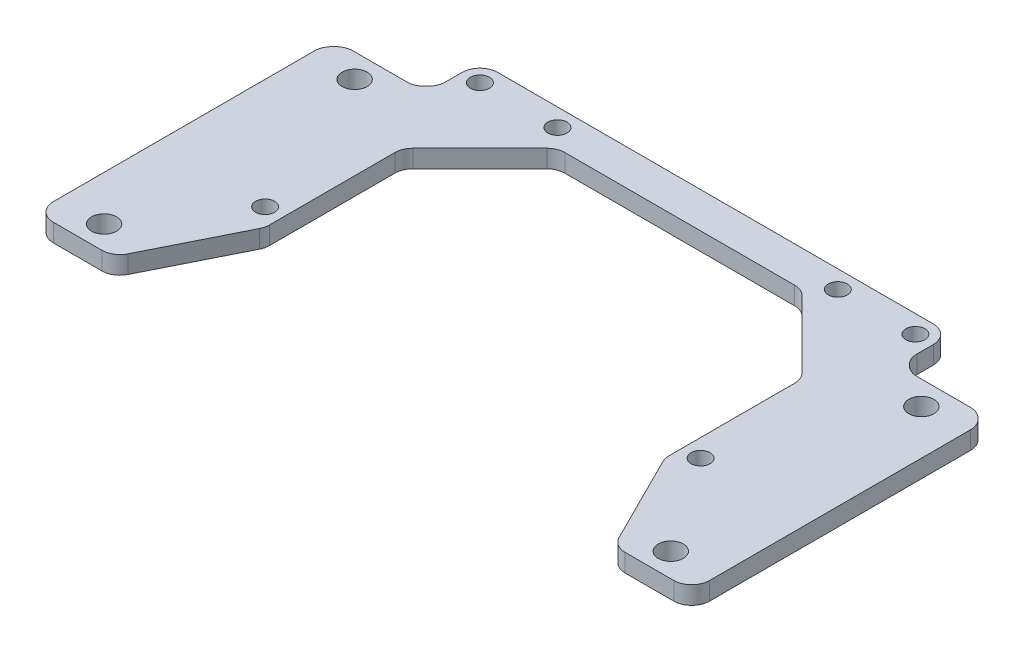
SolidWorks part; units mm, degrees
material "哈碳纤"
ref_plane "前视基准面" through (0, 0, 0) normal (0, 0, 1) x (1, 0, 0)
ref_plane "上视基准面" through (0, 0, 0) normal (0, 1, 0) x (1, 0, 0)
ref_plane "右视基准面" through (0, 0, 0) normal (1, 0, 0) x (0, 0, -1)
other "Configuration Table"
sketch "草图1" plane through (0, 0, 0) normal (0, 1, 0) x (1, 0, 0)
  line L0 (-23.5, 31) -> (23.5, 31) construction
  line L2 (-55, -25) -> (-55, 25)
  line L4 (55, -25) -> (55, 25)
  line L5 (-55, -25) -> (55, 25) construction
  line L6 (-55, 25) -> (55, -25) construction
  line L7 (-47.5, -21) -> (47.5, -21) construction
  line L8 (-47.5, -21) -> (-47.5, 21) construction
  line L9 (-47.5, 21) -> (47.5, 21) construction
  line L10 (47.5, -21) -> (47.5, 21) construction
  line L11 (-47.5, -21) -> (47.5, 21) construction
  line L12 (-47.5, 21) -> (47.5, -21) construction
  line L13 (-36.5, -5) -> (36.5, -5) construction
  line L14 (-36.5, -5) -> (-36.5, 31) construction
  line L15 (-36.5, 31) -> (36.5, 31) construction
  line L16 (36.5, -5) -> (36.5, 31) construction
  line L17 (-36.5, -5) -> (36.5, 31) construction
  line L18 (-36.5, 31) -> (36.5, -5) construction
  line L19 (0, -1000) -> (0, 49000) construction
  line L20 (-55, 25) -> (-39.5, 25)
  line L21 (55, 25) -> (39.5, 25)
  line L22 (-39.5, 25) -> (-39.5, 34)
  line L23 (39.5, 25) -> (39.5, 34)
  line L24 (-39.5, 34) -> (39.5, 34)
  line L25 (-55, -25) -> (-42, -25)
  line L26 (55, -25) -> (42, -25)
  line L27 (-42, -25) -> (-33.5, -8)
  line L28 (42, -25) -> (33.5, -8)
  line L29 (-33.5, -8) -> (-33.5, 28)
  line L30 (33.5, -8) -> (33.5, 28)
  line L31 (-33.5, 28) -> (0, 28)
  line L32 (33.5, 28) -> (0, 28)
  circle A0 centre (-47.5, 21) radius 2.1
  circle A1 centre (-47.5, -21) radius 2.1
  circle A2 centre (47.5, -21) radius 2.1
  circle A3 centre (47.5, 21) radius 2.1
  circle A4 centre (-36.5, 31) radius 1.6
  circle A5 centre (-36.5, -5) radius 1.6
  circle A6 centre (36.5, -5) radius 1.6
  circle A7 centre (36.5, 31) radius 1.6
  circle A8 centre (-23.5, 31) radius 1.6
  circle A9 centre (23.5, 31) radius 1.6
  point P0 (0, 0)
  point P5 (0, 0)
  point P15 (0, 13)
  point P28 (0, 31)
  point P36 (0, 34)
  dimension "D3" = 4.2
  dimension "D4" = 95
  dimension "D6" = 3.2
  dimension "D7" = 36
  dimension "D9" = 47
  dimension "D1" = 50
  dimension "D2" = 110
  dimension "D5" = 42
  dimension "D8" = 73
  dimension "D10" = 13
  dimension "D11" = 3
  dimension "D12" = 3
  dimension "D13" = 3
  dimension "D14" = 3
  dimension "D15" = 13
  dimension "D16" = 3
extrude "凸台-拉伸1" add sketch "草图1" along normal blind 3
chamfer "倒角1" distance 13 angle 45 2 edges at (33.5, 1.5, -28) (-33.5, 1.5, -28)
chamfer "倒角2" distance 2 angle 45 4 edges at (55, 1.5, -25) (39.5, 1.5, -25) (-55, 1.5, -25) (-39.5, 1.5, -25)
fillet "圆角1" radius 3 20 edges at (55, 1.5, 25) (42, 1.5, 25) (33.5, 1.5, 8) (33.5, 1.5, -15) (20.5, 1.5, -28) (-33.5, 1.5, -15) (-33.5, 1.5, 8) (-42, 1.5, 25) (-55, 1.5, 25) (-20.5, 1.5, -28) (-53, 1.5, -25) (-41.5, 1.5, -25) (41.5, 1.5, -25) (53, 1.5, -25) (55, 1.5, -23) (-55, 1.5, -23) (39.5, 1.5, -34) (-39.5, 1.5, -34) (-39.5, 1.5, -27) (39.5, 1.5, -27)
